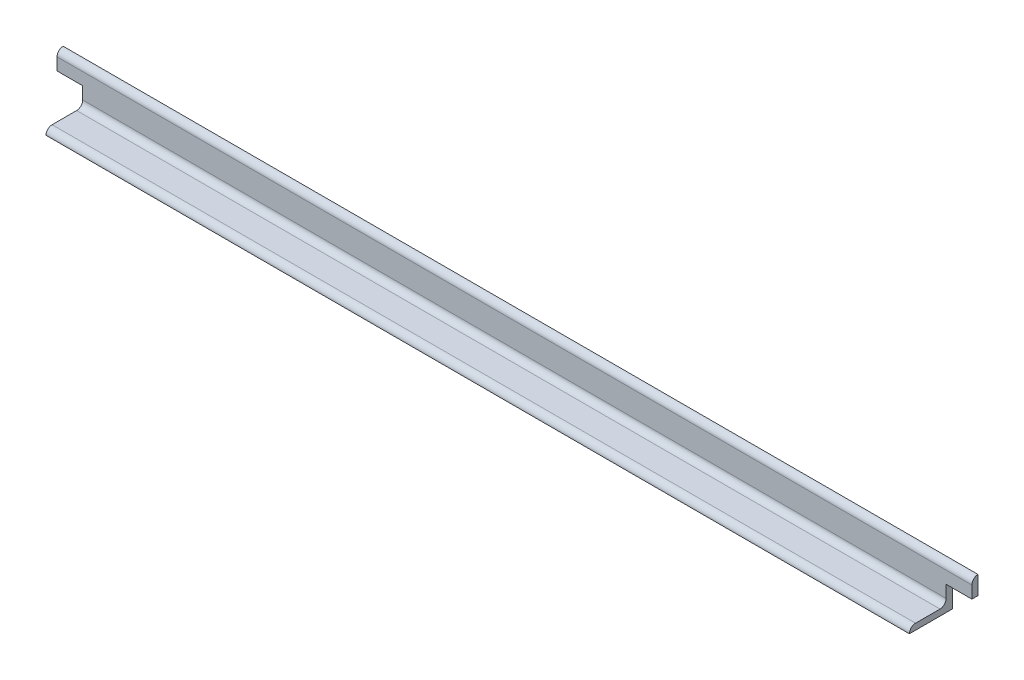
SolidWorks part; units mm, degrees
ref_plane "Front Plane" through (0, 0, 0) normal (0, 0, 1) x (1, 0, 0)
ref_plane "Top Plane" through (0, 0, 0) normal (0, 1, 0) x (1, 0, 0)
ref_plane "Right Plane" through (0, 0, 0) normal (1, 0, 0) x (0, 0, -1)
sketch "Sketch1" plane through (0, 0, 0) normal (0, 0, 1) x (1, 0, 0)
  line L0 (0, 0) -> (747, 0)
  dimension "D1" = 747
other "Angle Iron 35 X 35 X 5(1)"
ref_plane "Plane1" through (0, 0, 0) normal (1, 0, 0) x (0, 1, 0)
sketch "Sketch11" plane through (0, 0, 0) normal (1, 0, 0) x (0, 1, 0)
  line L0 (0, 0) -> (0, 35)
  line L1 (0, 17.5) -> (5, 17.5) construction
  line L2 (5, 30) -> (5, 10)
  line L3 (10, 5) -> (30, 5)
  line L4 (17.5, 5) -> (17.5, 0) construction
  line L5 (35, 0) -> (0, 0)
  arc A0 (35, 0) -> (30, 5) centre (30, 0) ccw
  arc A1 (0, 35) -> (5, 30) centre (0, 30) cw
  arc A2 (10, 5) -> (5, 10) centre (10, 10) cw
  point P10 (17.5, 0)
  point P14 (0, 17.5)
  point P15 (5, 17.5)
  point P16 (17.5, 5)
  point P17 (5, 35)
  point P18 (35, 5)
  point P21 (0, 0)
  dimension "D2" = 5
  dimension "D3" = 35
  dimension "Radius_1" = 5
  dimension "D1" = 5
sketch "Sketch2" plane through (0, 0, 0) normal (0, 0, -1) x (-1, 0, 0)
  line L0 (-373.5, 35) -> (-373.5, -78.0986) construction
  line L1 (0, 0) -> (-21, 0)
  line L2 (0, 0) -> (0, 20)
  line L3 (0, 20) -> (-21, 20)
  line L4 (-21, 0) -> (-21, 20)
  line L5 (-747, 35) -> (0, 35) construction
  line L6 (-726, 0) -> (-726, 20)
  line L7 (-747, 20) -> (-726, 20)
  line L8 (-747, 0) -> (-747, 20)
  line L9 (-747, 0) -> (-726, 0)
  dimension "D1" = 21
  dimension "D2" = 20
extrude "Cut-Extrude1" cut sketch "Sketch2" against normal through all contours L4 L3 L2 L1
